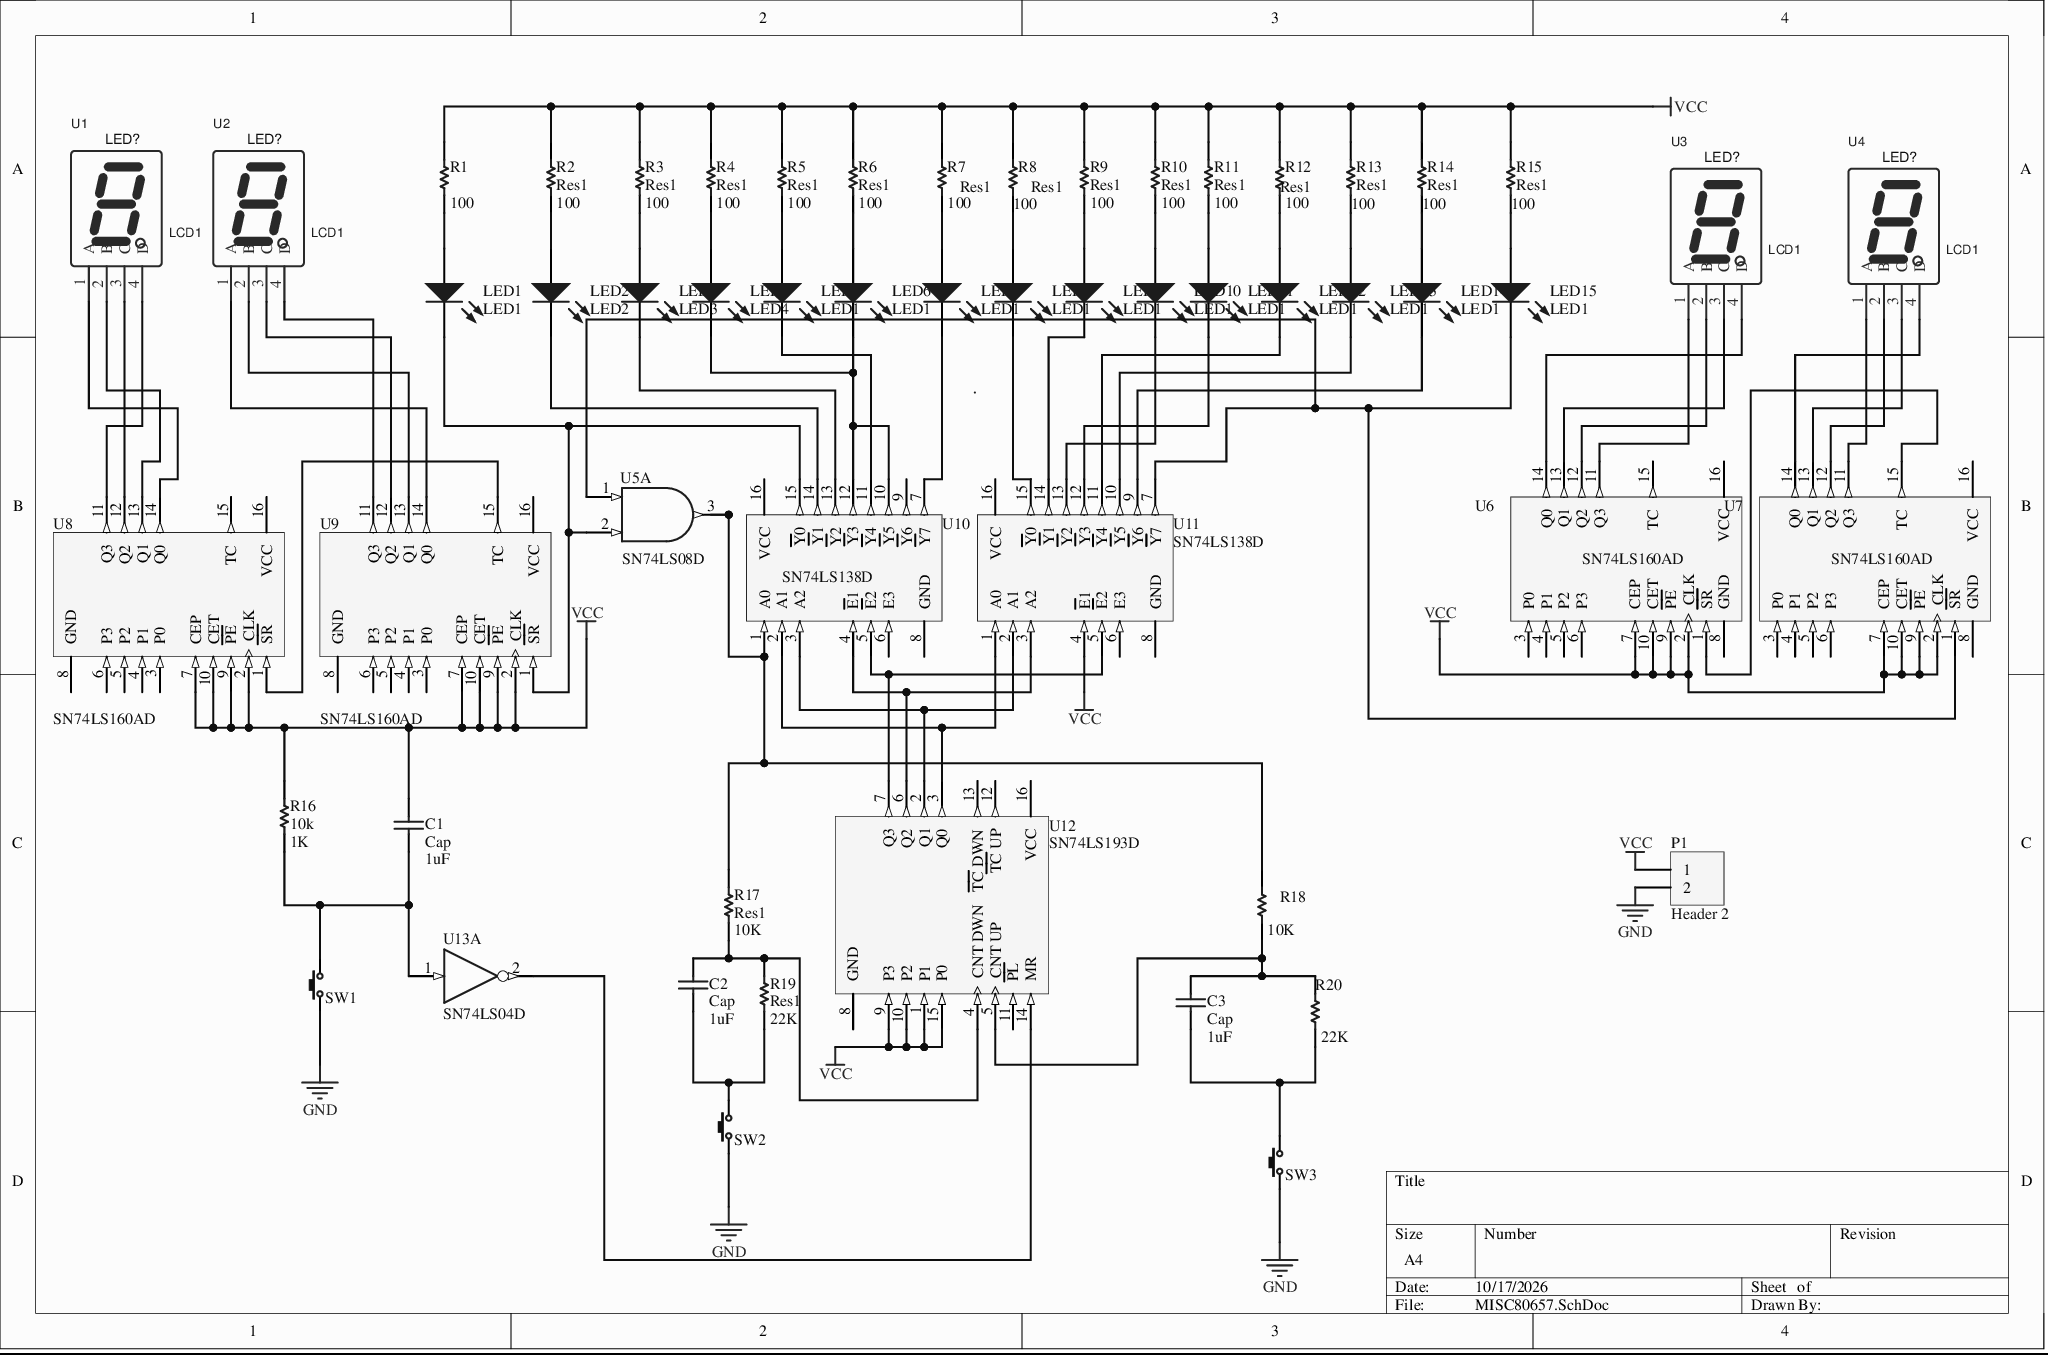
[diagram p0: MISC80657.SchDoc]
# Altium project MISC80657.PrjPcb
1 sheet, 55 parts. Net scope: global (net labels, ports and power ports of the same name join across sheets).
Board file: MISC80657.PcbDoc

## Sheet MISC80657.SchDoc
size A4

### Parts
C1  Cap  value 1uF  [CS 2.0*5*8 - C]
C2  Cap  value 1uF  [CS 2.0*5*8 - C]
C3  Cap  value 1uF  [CS 2.0*5*8 - C]
LED1  LED1  [LED 3MM-B]
LED2  LED2  [LED 3MM-B]
LED3  LED3  [LED 3MM-B]
LED4  LED4  [LED 3MM-B]
LED5  LED1  [LED 3MM-B]
LED6  LED1  [LED 3MM-B]
LED7  LED1  [LED 3MM-B]
LED8  LED1  [LED 3MM-B]
LED9  LED1  [LED 3MM-B]
LED10  LED1  [LED 3MM-B]
LED11  LED1  [LED 3MM-B]
LED12  LED1  [LED 3MM-B]
LED13  LED1  [LED 3MM-B]
LED14  LED1  [LED 3MM-B]
LED15  LED1  [LED 3MM-B]
P1  Header 2  [HDR1X2]
R1  value 100  [RS 1/4W]
R2  Res1  value 100  [RS 1/4W]
R3  Res1  value 100  [RS 1/4W]
R4  Res1  value 100  [RS 1/4W]
R5  Res1  value 100  [RS 1/4W]
R6  Res1  value 100  [RS 1/4W]
R7  Res1  value 100  [RS 1/4W]
R8  Res1  value 100  [RS 1/4W]
R9  Res1  value 100  [RS 1/4W]
R10  Res1  value 100  [RS 1/4W]
R11  Res1  value 100  [RS 1/4W]
R12  Res1  value 100  [RS 1/4W]
R13  Res1  value 100  [RS 1/4W]
R14  Res1  value 100  [RS 1/4W]
R15  Res1  value 100  [RS 1/4W]
R16  10k  value 1K  [RS 1/4W]
R17  Res1  value 10K  [RS 1/4W]
R18  value 10K  [RS 1/4W]  (hidden comment: Res1)
R19  Res1  value 22K  [RS 1/4W]
R20  value 22K  [RS 1/4W]
SW1  3x6x5  [TSW DIP-3*6*4.3]  (value not drawn)
SW2  3x6x5  [TSW DIP-3*6*4.3]  (value not drawn)
SW3  3x6x5  [TSW DIP-3*6*4.3]  (value not drawn)
U1  LCD1  [DCD-HEX]
U2  LCD1  [DCD-HEX]
U3  LCD1  [DCD-HEX]
U4  LCD1  [DCD-HEX]
U5  SN74LS08D  [DIP14]  (part A of 4)
U6  SN74LS160AD  [DIP16]
U7  SN74LS160AD  [DIP16]
U8  SN74LS160AD  [DIP16]
U9  SN74LS160AD  [DIP16]
U10  SN74LS138D  [DIP16]
U11  SN74LS138D  [DIP16]
U12  SN74LS193D  [DIP16]
U13  SN74LS04D  [DIP14]  (part A of 6)

### Nets
GND: P1.2 SW1.1 SW2.1 SW3.1 U5.7(GND) U13.7(GND)
VCC: C1.2 P1.1 R1.2 R2.2 R3.2 R4.2 R5.2 R6.2 R7.2 R8.2 R9.2 R10.2 R11.2 R12.2 R13.2 R14.2 R15.2 R16.2 U5.14(VCC) U6.2(CLK) U6.7(CEP) U6.9(~{PE}) U6.10(CET) U7.2(CLK) U7.7(CEP) U7.9(~{PE}) U7.10(CET) U8.2(CLK) U8.7(CEP) U8.9(~{PE}) U8.10(CET) U9.2(CLK) U9.7(CEP) U9.9(~{PE}) U9.10(CET) U11.4(~{E}1) U12.1(P1) U12.9(P3) U12.10(P2) U12.15(P0)
VDD: U13.14(VDD)
NetC1_1: C1.1 R16.1 SW1.2 U13.1(IN)
NetC2_1: C2.1 R19.1 SW2.2
NetC2_2: C2.2 R17.1 R19.2 U12.4(CNT_DWN)
NetC3_1: C3.1 R20.1 SW3.2
NetC3_2: C3.2 R18.1 R20.2 U12.5(CNT_UP)
NetLED1_1: LED1.1(A) R1.1
NetLED1_2: LED1.2(K) U5.2(B) U9.1(~{SR}) U10.15(~{Y}0)
NetLED2_1: LED2.1(A) R2.1
NetLED2_2: LED2.2(K) U10.14(~{Y}1)
NetLED3_1: LED3.1(A) R3.1
NetLED3_2: LED3.2(K) U10.13(~{Y}2)
NetLED4_1: LED4.1(A) R4.1
NetLED4_2: LED4.2(K) LED6.2(K) U10.10(~{Y}5) U10.12(~{Y}3)
NetLED5_1: LED5.1(A) R5.1
NetLED5_2: LED5.2(K) U10.11(~{Y}4)
NetLED6_1: LED6.1(A) R6.1
NetLED7_1: LED7.1(A) R7.1
NetLED7_2: LED7.2(K) U10.7(~{Y}7)
NetLED8_1: LED8.1(A) R8.1
NetLED8_2: LED8.2(K) U11.15(~{Y}0)
NetLED9_1: LED9.1(A) R9.1
NetLED9_2: LED9.2(K) U11.14(~{Y}1)
NetLED10_1: LED10.1(A) R10.1
NetLED10_2: LED10.2(K) U11.13(~{Y}2)
NetLED11_1: LED11.1(A) R11.1
NetLED11_2: LED11.2(K) U11.12(~{Y}3)
NetLED12_1: LED12.1(A) R12.1
NetLED12_2: LED12.2(K) U11.11(~{Y}4)
NetLED13_1: LED13.1(A) R13.1
NetLED13_2: LED13.2(K) U11.10(~{Y}5)
NetLED14_1: LED14.1(A) R14.1
NetLED14_2: LED14.2(K) U11.9(~{Y}6)
NetLED15_1: LED15.1(A) R15.1
NetLED15_2: LED15.2(K) U5.1(A) U7.1(~{SR}) U11.7(~{Y}7)
NetR17_2: R17.2 R18.2 U5.3(Y) U10.1(A0)
NetU1_1: U1.1(A) U8.14(Q0)
NetU1_2: U1.2(B) U8.13(Q1)
NetU1_3: U1.3(C) U8.12(Q2)
NetU1_4: U1.4(D) U8.11(Q3)
NetU2_1: U2.1(A) U9.14(Q0)
NetU2_2: U2.2(B) U9.13(Q1)
NetU2_3: U2.3(C) U9.12(Q2)
NetU2_4: U2.4(D) U9.11(Q3)
NetU3_1: U3.1(A) U6.11(Q3)
NetU3_2: U3.2(B) U6.12(Q2)
NetU3_3: U3.3(C) U6.13(Q1)
NetU3_4: U3.4(D) U6.14(Q0)
NetU4_1: U4.1(A) U7.11(Q3)
NetU4_2: U4.2(B) U7.12(Q2)
NetU4_3: U4.3(C) U7.13(Q1)
NetU4_4: U4.4(D) U7.14(Q0)
NetU6_1: U6.1(~{SR}) U7.15(TC)
NetU8_1: U8.1(~{SR}) U9.15(TC)
NetU10_2: U10.2(A1) U11.1(A0) U12.3(Q0)
NetU10_3: U10.3(A2) U11.2(A1) U12.2(Q1)
NetU10_4: U10.4(~{E}1) U11.3(A2) U12.6(Q2)
NetU10_5: U10.5(~{E}2) U11.5(~{E}2) U12.7(Q3)
NetU12_14: U12.14(MR) U13.2(~{OUT})

Not connected (* = marked no-connect by the designer): U6 3(P0) 4(P1) 5(P2) 6(P3) 8(GND) 15(TC) 16(VCC); U7 3(P0) 4(P1) 5(P2) 6(P3) 8(GND) 16(VCC); U8 3(P0) 4(P1) 5(P2) 6(P3) 8(GND) 15(TC) 16(VCC); U9 3(P0) 4(P1) 5(P2) 6(P3) 8(GND) 16(VCC); U10 6(E3) 8(GND) 9(~{Y}6) 16(VCC); U11 6(E3) 8(GND) 16(VCC); U12 8(GND) 11(~{PL}) 12(~{TC}_UP) 13(~{TC}_DWN) 16(VCC)

### Library data of the parts
C1-C3 = Cap: Capacitor; Published: 8-Jun-2000; LatestRevisionDate: 17-Jul-2002; LatestRevisionNote: Re-released for DXP Platform.; PackageReference: RAD-0.3; PackageDescription: Radial Cap, Thru-Hole; 2 Leads; 0.3 in Pin Spacing; Publisher: Altium Limited
LED1-LED15 = LED3: Typical BLUE SiC LED; Published: 8-Jun-2000; LatestRevisionDate: 17-Dec-2003; LatestRevisionNote: PCB Footprint replaced.; DatasheetVersion: 16-Apr-2002; PackageVersion: 16-Apr-2002; PackageReference: 3.5X2.8X1.9; PackageDescription: SM LED; 2 C-Bend Leads; Body 3.5 x 2.8 x 1.9 mm, inc leads (LxWxH typ); Publisher: Altium Limited
P1 = Header 2: Header, 2-Pin; LatestRevisionDate: 17-Jul-2002; LatestRevisionNote: Re-released for DXP Platform.; Publisher: Altium Limited
R1-R20 = Res1: Resistor; Published: 8-Jun-2000; LatestRevisionDate: 17-Jul-2002; LatestRevisionNote: Re-released for DXP Platform.; PackageReference: AXIAL-0.3; PackageDescription: Axial Device, Thru-Hole; 2 Leads; 0.3 in Pin Spacing; Publisher: Altium Limited
SW1-SW3 = TSW 3x6: 3x6 tactile switch; BOM名称: 3x6 tactile switch
U5 = SN74LS08D: Quad 2-Input AND Gate; Code - JEDEC: MS-012-AB; Code - IPC: SO14; Published: 15-Apr-2002; Datasheet: Latest Revision: Dec-1999; Package Reference: 751A-03; Publisher: Altium Limited
U6-U9 = SN74LS160AD: BCD Decade Counter; Package Information: Latest Revision: 1991; Code - JEDEC: MS-012-AC; Code - IPC: SO16; Published: 15-Apr-2002; Datasheet: Latest Revision: 18-Oct-1996; Package Reference: 751B-03; Publisher: Altium Limited
U10 U11 = SN74LS138D: 1-of-8 Decoder/Demultiplexer; Package Information: Latest Revision: Oct-1999; Code - JEDEC: MS-012-AC; Code - IPC: SO16; Published: 15-Apr-2002; Datasheet: Latest Revision: Dec-1999; Package Reference: 751B-05; Publisher: Altium Limited
U12 = SN74LS193D: Presettable 4-Bit Binary Up/Down Counter; Package Information: Latest Revision: 1991; Code - JEDEC: MS-012-AC; Code - IPC: SO16; Published: 15-Apr-2002; Datasheet: Latest Revision: 18/10/1996; Package Reference: 751B-03; Publisher: Altium Limited
U13 = SN74LS04D: Hex Inverter; Code - JEDEC: MS-012-AB; Code - IPC: SO14; Published: 15-Apr-2002; Datasheet: Latest Revision: 1999; Package Reference: 751A-03; Publisher: Altium Limited